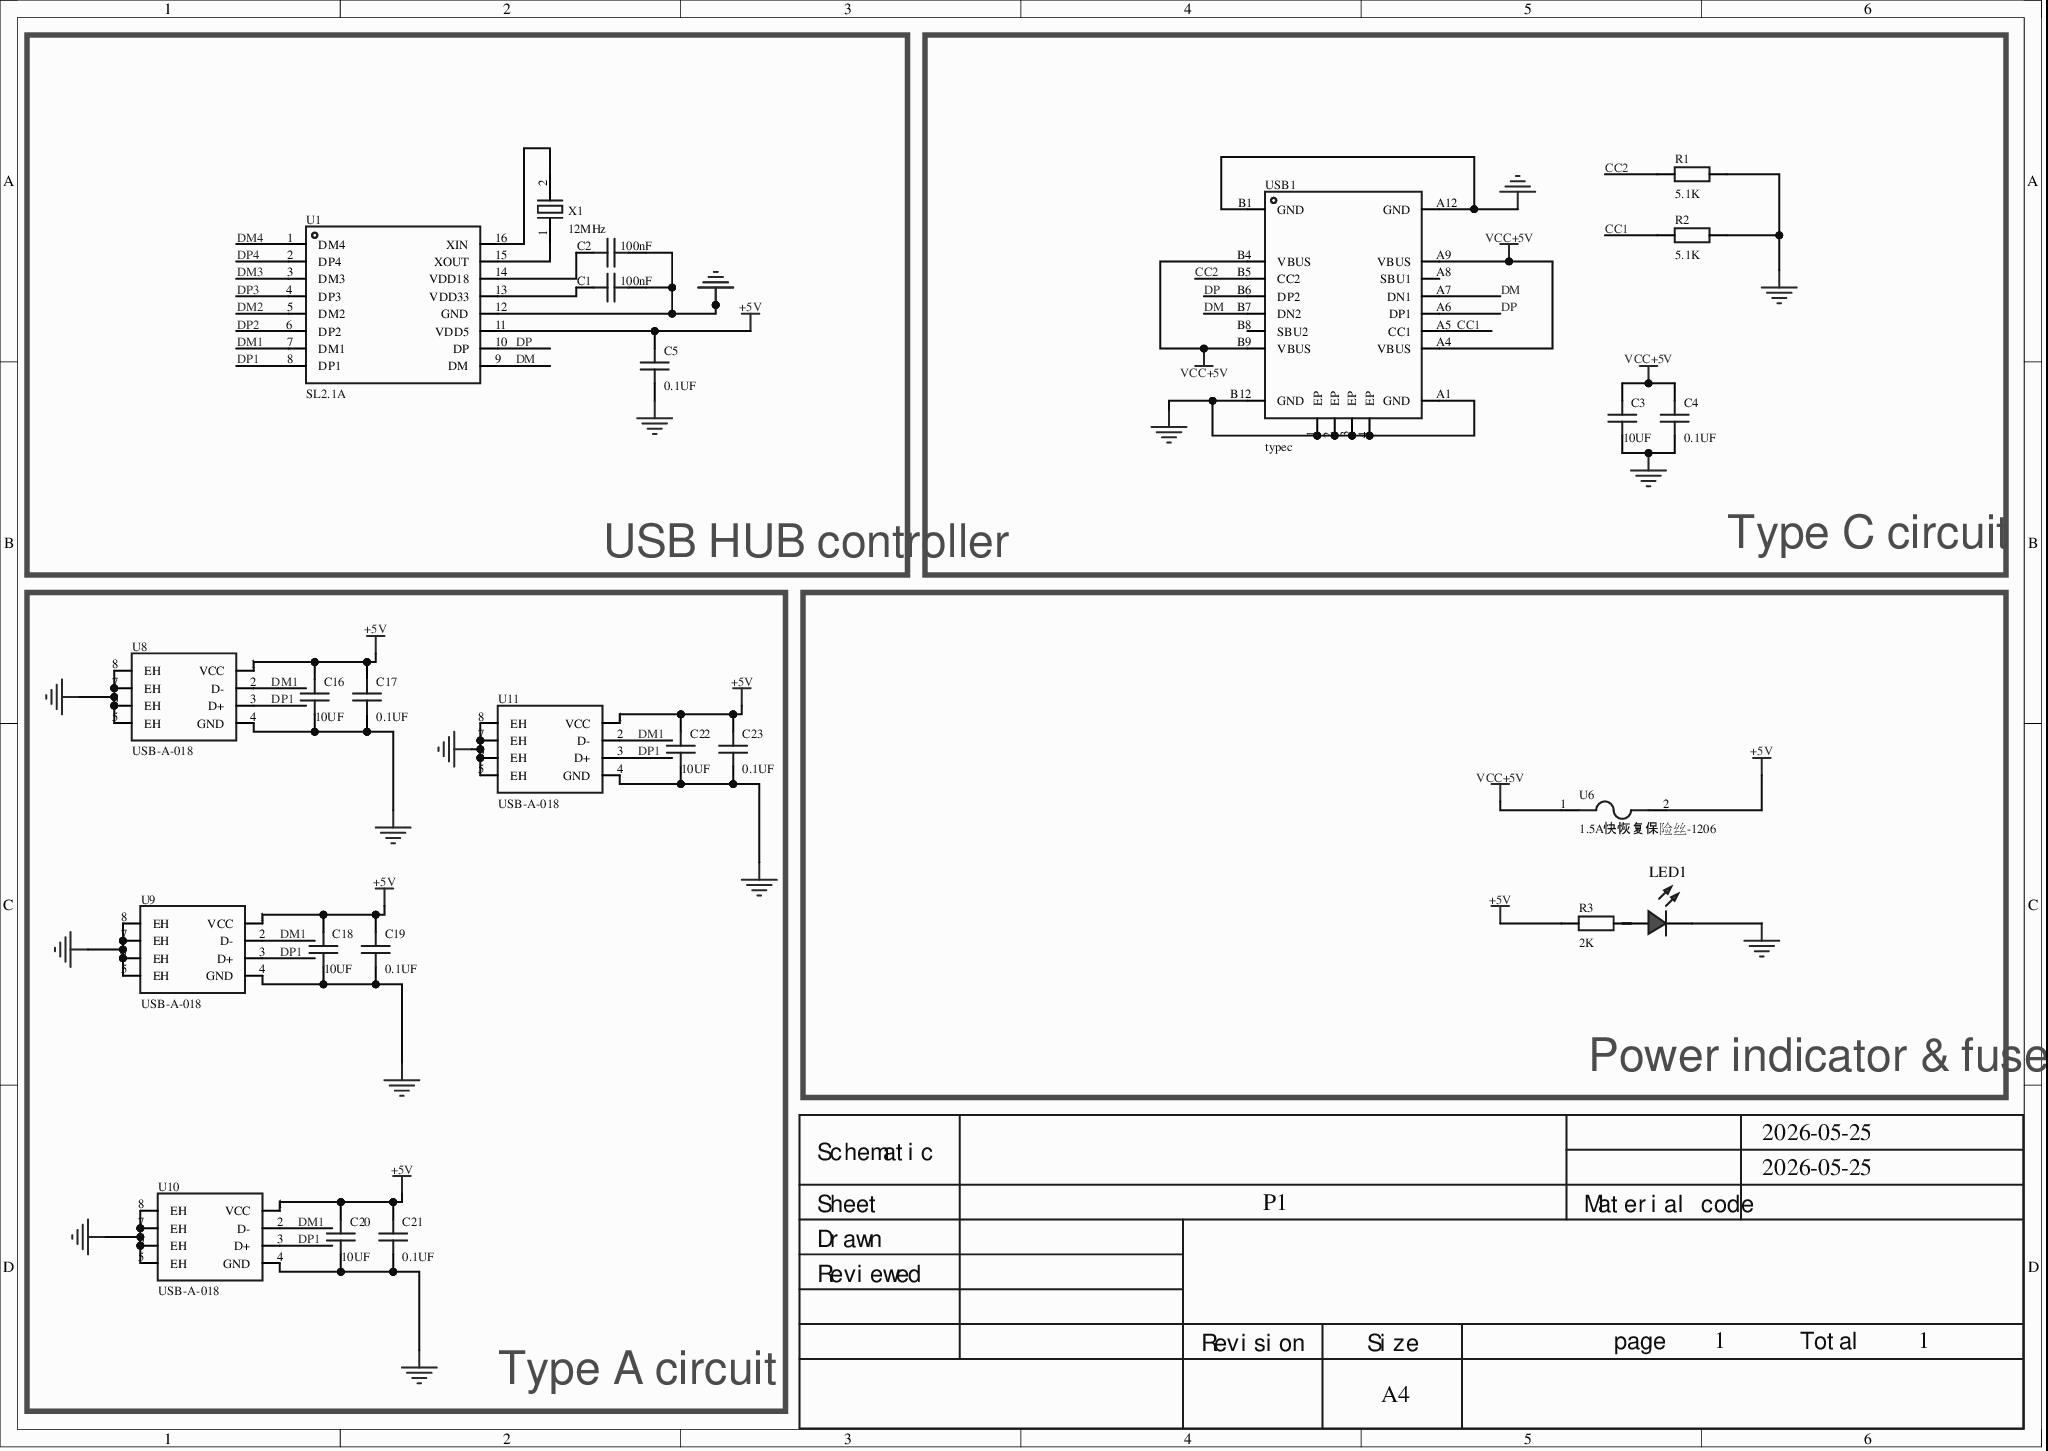
[diagram p0: MISC51874-3.schdoc]
# Altium project MISC51874-2.PrjPcb
1 sheet, 25 parts. Net scope: global (net labels, ports and power ports of the same name join across sheets).
Board file: MISC51874.pcbdoc

## Sheet MISC51874-3.schdoc
size 297 x 210 mm; Version: V1.0; @Project Name: MISC51874; @Page Count: 1; @Update Date: 2026-05-25; @Create Date: 2026-05-25; @Schematic Name: MISC51874; @Page No: 1

### Parts
C1  100nF  [C0805]
C2  100nF  [C0805]
C3  10UF  [C0805]
C4  0.1UF  [C0805]
C5  0.1UF  [C0805]
C16  10UF  [C0805]
C17  0.1UF  [C0805]
C18  10UF  [C0805]
C19  0.1UF  [C0805]
C20  10UF  [C0805]
C21  0.1UF  [C0805]
C22  10UF  [C0805]
C23  0.1UF  [C0805]
LED1  (no value)  [LED_0805]
R1  5.1K  [R0805]
R2  5.1K  [R0805]
R3  2K  [R0805]
U1  SL2.1A  [SOP-16_L10.0-W3.9-P1.27-LS6.0-BL]
U6  1.5A快恢复保险丝-1206  [F1206]
U8  USB-A-018  [usb-smd_usb-a-018]
U9  USB-A-018  [usb-smd_usb-a-018]
U10  USB-A-018  [usb-smd_usb-a-018]
U11  USB-A-018  [usb-smd_usb-a-018]
USB1  typec  [USB-C-SMD_KH-TYPE-C-16P]
X1  12MHz  [CRYSTAL-SMD_L11.1-W4.8-LS12.3]

### Blocks framed on the sheet
USB HUB controller: C1 C2 C5 U1 X1
Type C circuit: C3 C4 R1 R2 USB1
Type A circuit: C16-C23 U8-U11
Power indicator & fuse: LED1 R3 U6

### Nets
+5V: C5.2 C16.2 C17.2 C18.2 C19.2 C20.2 C21.2 C22.2 C23.2 R3.2 U1.11(VDD5) U6.2 U8.1(VCC) U9.1(VCC) U10.1(VCC) U11.1(VCC)
GND: C1.2 C2.2 C3.1 C4.1 C5.1 C16.1 C17.1 C18.1 C19.1 C20.1 C21.1 C22.1 C23.1 LED1.1(C) R1.2 R2.2 U1.12(GND) U8.4(GND) U8.5(EH) U8.6(EH) U8.7(EH) U8.8(EH) U9.4(GND) U9.5(EH) U9.6(EH) U9.7(EH) U9.8(EH) U10.4(GND) U10.5(EH) U10.6(EH) U10.7(EH) U10.8(EH) U11.4(GND) U11.5(EH) U11.6(EH) U11.7(EH) U11.8(EH) USB1.1(EP) USB1.2(EP) USB1.3(EP) USB1.4(EP) USB1.A1(GND) USB1.A12(GND) USB1.B1(GND) USB1.B12(GND)
VCC+5V: C3.2 C4.2 U6.1 USB1.A4(VBUS) USB1.A9(VBUS) USB1.B4(VBUS) USB1.B9(VBUS)
CC1: R2.1 USB1.A5(CC1)
CC2: R1.1 USB1.B5(CC2)
DM: U1.9(DM) USB1.A7(DN1) USB1.B7(DN2)
DM1: U1.7(DM1) U8.2(D-) U9.2(D-) U10.2(D-) U11.2(D-)
DM2: U1.5(DM2)
DM3: U1.3(DM3)
DM4: U1.1(DM4)
DP: U1.10(DP) USB1.A6(DP1) USB1.B6(DP2)
DP1: U1.8(DP1) U8.3(D+) U9.3(D+) U10.3(D+) U11.3(D+)
DP2: U1.6(DP2)
DP3: U1.4(DP3)
DP4: U1.2(DP4)
NetC1_1: C1.1 U1.13(VDD33)
NetC2_1: C2.1 U1.14(VDD18)
NetLED1_2: LED1.2(A) R3.1
NetU1_15: U1.15(XOUT) X1.1
NetU1_16: U1.16(XIN) X1.2(GND)

Not connected (* = marked no-connect by the designer): USB1 A8(SBU1)* B8(SBU2)*

### Notes on the sheet
- 2026-05-25
- Schematic
- Sheet
- P1
- Material code
- Reviewed
- Drawn
- Revision
- Size
- A4
- page
- 1
- Total

### Library data of the parts
C1-C5 C16-C23 = CAP_0805: ConvertToPcb: yes; SymbolName: CapAcitance; ModelId: 1ba041120af144c991958decab20d241; ModelName: C0805_L2.0-W1.3-H1.3; ModelTransform: 78.74,51.181,0,0,0,0,0,0.0005,0; Device: CAP_0805; AddInBom: yes; Supplier Footprint: 0805; FootprintName: C0805
  C1 C2: Value: 100nF
  C3 C16 C18 C20 C22: Value: 10UF
  C4 C5 C17 C19 C21 C23: Value: 0.1UF
LED1 = LED_0805-R: Symbol: LED_R; Convert to PCB: yes; 3D Model: 33fb9fca58e84f37a403ebeef4c28b77; 3D Model Transform: 78.7,49.1,39.3,0,0,0,0,0,0; ModelName: LED-0805_R; Device: LED_0805-R; Add into BOM: yes; Supplier Footprint: 0805; FootprintName: LED_0805
R1-R3 = Res_0805: Symbol: Resistor; ConvertToPcb: yes; ModelId: 37a81e68749a4138bd2dfa6897b24b85; ModelName: R0805_L2.0-W1.3-H0.6; ModelTransform: 78.74,51.181,0,0,0,0,0,-0.0005,0; Device: Res_0805; AddInBom: yes; Supplier Footprint: 0805; FootprintName: R0805
  R1 R2: Value: 5.1K
  R3: Value: 2K
U1 = SL2.1A: Application function: hub; interface protocol: -;; Manufacturer: CoreChips(和芯润德); AddInBom: yes; ModelId: 3361a6792abf4a8f8fbca4f1924a67ee; ModelName: SOP-16_L9.9-W3.9-H1.5-LS6.0-P1.27; ModelTransform: 240.39054,393.7,0,90,0,0,0,0,0; Symbol: SL2.1A; Device: SL2.1A; LCSC Part Name: SL2.1A USB2.0 HUB 控制器集成电路; SupplierPart: C192893; ManufacturerPart: SL2.1A; Supplier Footprint: SOP-16; JLCPCB Part Class: Extended library; Datasheet: https://atta.szlcsc.com/upload/public/pdf/source/20180522/C192893_624110D24898D57AAC785E3DF98EA862.pdf; Supplier: LCSC; ConvertToPcb: yes; FootprintName: SOP-16_L10.0-W3.9-P1.27-LS6.0-BL; Applications Function: Hub; Protocol: -
U6 = 1.5A快恢复保险丝-1206: AddInBom: yes; ModelId: f1628daad26847a79b887277a2bc8541; ModelName: F1206_L3.2-W1.7-H0.6; ModelTransform: 125.984,66.929,0,0,0,0,0,0,0; Symbol: 1.5A快恢复保险丝-1206; Device: 1.5A快恢复保险丝-1206; LCSC Part Name: 1.5A快恢复保险丝-1206; SupplierPart: C9900012139; ManufacturerPart: 1.5A快恢复保险丝-1206; Supplier Footprint: F1206; JLCPCB Part Class: Extended library; Supplier: LCSC; ConvertToPcb: yes; FootprintName: F1206
U8-U11 = USB-A-018: AddInBom: yes; ModelId: aeefe6e3ae3240d7a5181a7beb45f4db; ModelTransform: 624.0145,482.28246,0,0,0,0,1.535,-102.085,-55.118; Symbol: USB-A-018; Device: USB-A-018; LCSC Part Name: USB-A-018; SupplierPart: C9900112287; ManufacturerPart: USB-A-018; Supplier Footprint: USB-4-SMT-DTCB; JLCPCB Part Class: Extended library; Supplier: LCSC; ConvertToPcb: yes; FootprintName: usb-smd_usb-a-018; ModelName: USB-SMD_USB-A-018
USB1 = typec: Symbol: TYPEC_C9900016956; AddInBom: yes; ModelId: f2c381012fbf47e0b76dea5162270f01; ModelTransform: 351.9678,307.48,0,0,0,0,0,-45.275,-43.307; Device: typec; LCSC Part Name: typec; SupplierPart: C9900016956; ManufacturerPart: typec; Supplier Footprint: typec 12p; JLCPCB Part Class: Extended library; Supplier: LCSC; ConvertToPcb: yes; FootprintName: USB-C-SMD_KH-TYPE-C-16P; ModelName: USB-C-SMD_KH-TYPE-C-16P
X1 = 9AT12000201060C3: Crystal type: SMD crystal; frequency: 12MHz; frequency tolerance at room temperature: ±10ppm; external load capacitance: 20pF;; Manufacturer: JGHC(晶光华); AddInBom: yes; ModelId: 5e1ead0cf76448b7a4ec480b96b3d6f4; ModelTransform: 484.251,190.1571,0,0,0,0,0,0,0; Equivalent Series Resistance (ESR): 60Ω; Symbol: 9AT12000201060C3; Device: 9AT12000201060C3; LCSC Part Name: 12MHz ±10ppm 20pF; SupplierPart: C2715880; ManufacturerPart: 9AT12000201060C3; Supplier Footprint: HC-49S-SMD; JLCPCB Part Class: Extended library; Datasheet: https://atta.szlcsc.com/upload/public/pdf/source/20210402/C2715880_322A8E636A60333B79E5FA4934B2EA11.pdf; Supplier: LCSC; ConvertToPcb: yes; FootprintName: CRYSTAL-SMD_L11.1-W4.8-LS12.3; ModelName: CRYSTAL-SMD_L11.1-W4.8-LS12.3; Crystal Type: SMD crystal; Value: 12MHz; Normal temperature Frequency Tolerance: ±10ppm; External load capacitor: 20pF; Operating Temperature: -40℃~+85℃